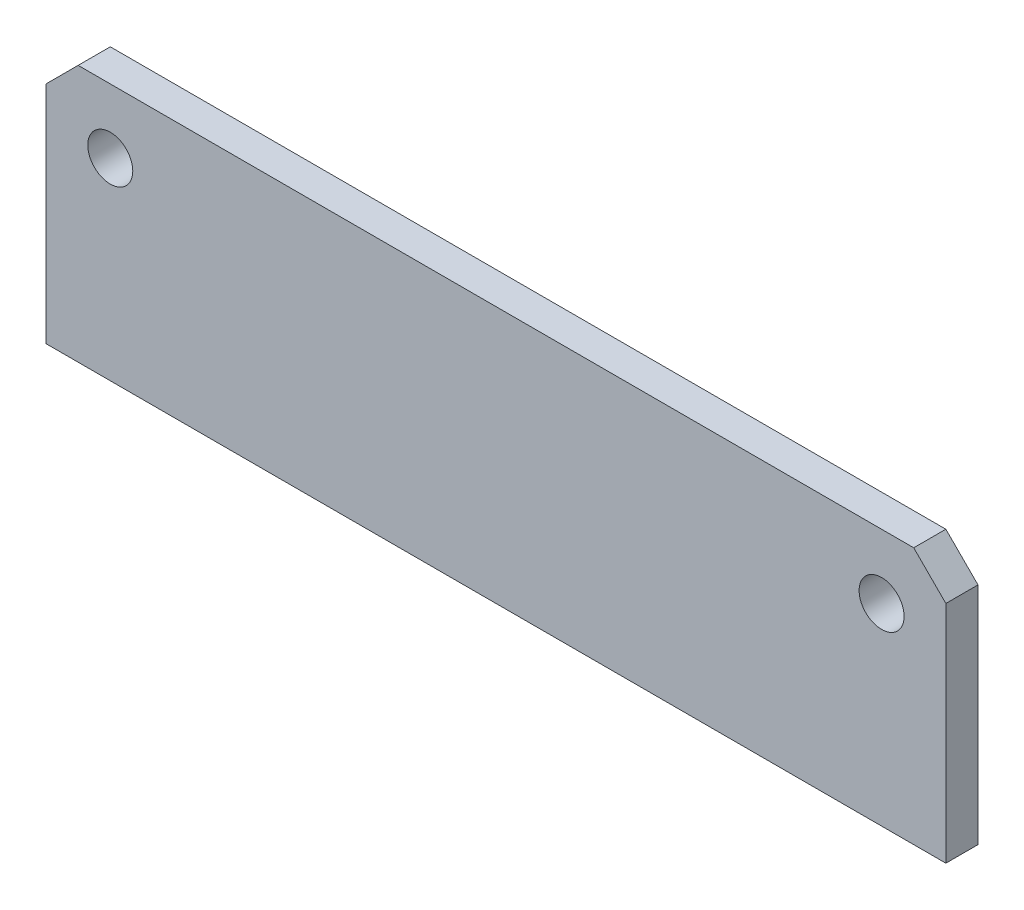
from build123d import *

# Parameters (mm, degrees)
SKETCH_1_W          = 140
SKETCH_1_H          = 40
EXTRUDE_1_DEPTH     = 5
SKETCH_2_R          = 3.5
CUT_EXTRUDE_1_DEPTH = 5
CHAMFER_1_SIZE      = 5


with BuildPart() as part:
    # 草图1 → 凸台-拉伸1 (new body)
    with BuildSketch(Plane.XY):
        Rectangle(SKETCH_1_W, SKETCH_1_H)
    extrude(amount=EXTRUDE_1_DEPTH)

    # 草图2 → 切除-拉伸1 (cut)
    with BuildSketch(Plane.XY.offset(5)):
        with Locations((-60, 10)):
            Circle(SKETCH_2_R)
        with Locations((60, 10)):
            Circle(SKETCH_2_R)
    extrude(amount=-CUT_EXTRUDE_1_DEPTH, mode=Mode.SUBTRACT)

    # 倒角1
    chamfer_1_edges = [part.edges().sort_by_distance(p)[0] for p in [
        (-70, 20, 2.5),
        (70, 20, 2.5),
    ]]
    chamfer(chamfer_1_edges, length=CHAMFER_1_SIZE)


solid = part.part
